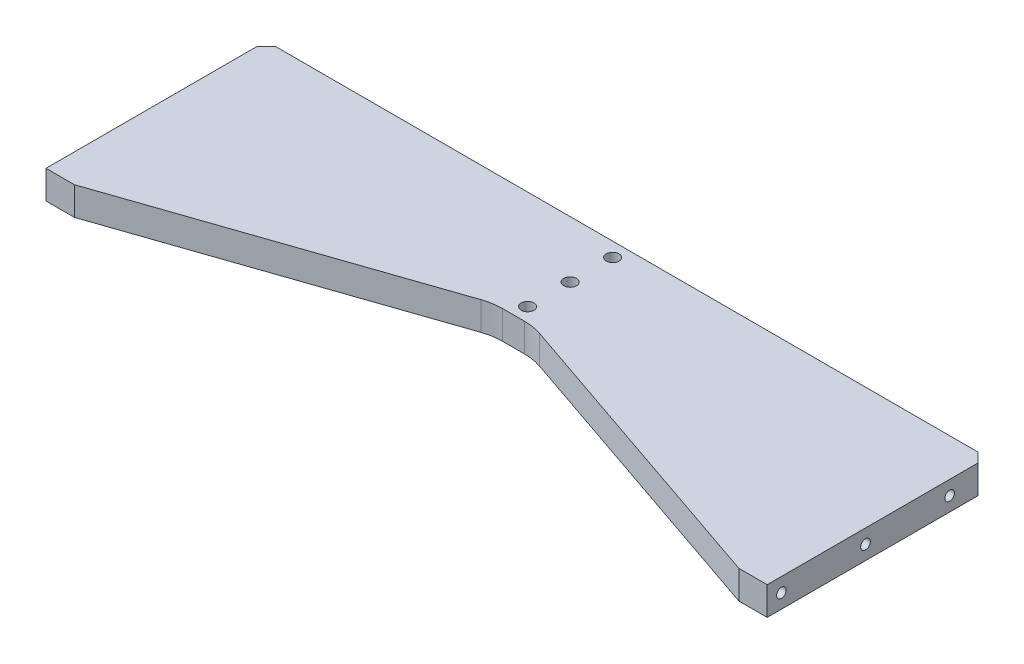
from build123d import *

# Parameters (mm, degrees)
SKETCH_1_W                = 763
SKETCH_1_H                = 233
EXTRUDE_1_DEPTH           = 30
CHAMFER_1_SIZE            = 10
CUT_EXTRUDE_1_DEPTH       = 401.018124589
CUT_EXTRUDE_1_DEPTH_BACK  = 30
FILLET_1_R                = 60
HOLE_WIZARD_1_D           = 13.5
HOLE_WIZARD_1_CBORE_D     = 20
HOLE_WIZARD_1_CBORE_DEPTH = 13
HOLE_WIZARD_M12_1_D       = 10.2
HOLE_WIZARD_M12_1_DEPTH   = 29.25
HOLE_WIZARD_M12_1_TIP     = 3.064389157
HOLE_WIZARD_M12_2_D       = 10.2
HOLE_WIZARD_M12_2_DEPTH   = 29.25
HOLE_WIZARD_M12_2_TIP     = 3.064389157
HOLE_WIZARD_M12_3_D       = 10.2
HOLE_WIZARD_M12_3_DEPTH   = 29.25
HOLE_WIZARD_M12_3_TIP     = 3.064389157


with BuildPart() as part:
    # 草图1 → 凸台-拉伸1 (new body)
    with BuildSketch(Plane(origin=(0, 0, 0), x_dir=(1, 0, 0), z_dir=(0, 1, 0))):
        Rectangle(SKETCH_1_W, SKETCH_1_H)
    extrude(amount=EXTRUDE_1_DEPTH)

    # 倒角1
    chamfer_1_edges = [part.edges().sort_by_distance(p)[0] for p in [
        (-381.5, 15, -116.5),
        (381.5, 15, -116.5),
    ]]
    chamfer(chamfer_1_edges, length=CHAMFER_1_SIZE)

    # 草图2 → 切除-拉伸1 (cut, two sides: drawn at the far end of the back side and taken through both)
    with BuildSketch(Plane(origin=(0, 30, 0), x_dir=(1, 0, 0), z_dir=(0, 1, 0)).offset(-CUT_EXTRUDE_1_DEPTH_BACK)):
        Polygon((-1816.285660926, -618.078120257), (-351.5, -116.5), (-21.5, -3.5), (21.5, -3.5), (351.5, -116.5), (1816.285660926, -618.078120257), (1816.285660926, -3714.642437803), (-1816.285660926, -3714.642437803), align=None)
    extrude(amount=CUT_EXTRUDE_1_DEPTH + CUT_EXTRUDE_1_DEPTH_BACK, mode=Mode.SUBTRACT)

    # 圆角1
    fillet_1_edges = [part.edges().sort_by_distance(p)[0] for p in [
        (21.5, 15, 3.5),
        (-21.5, 15, 3.5),
    ]]
    fillet(fillet_1_edges, radius=FILLET_1_R)

    # 打孔尺寸(%根据)内六角圆柱头螺钉的类型1 (through all)
    with Locations(Plane(origin=(0, 0, 0), x_dir=(-1, 0, 0), z_dir=(0, -1, 0))):
        with Locations((0, 11.5), (0, 56.5), (0, 101.5)):
            CounterBoreHole(HOLE_WIZARD_1_D / 2, HOLE_WIZARD_1_CBORE_D / 2, HOLE_WIZARD_1_CBORE_DEPTH)

    # M12 螺纹孔1
    with Locations(Plane(origin=(0, 0, -116.5), x_dir=(-1, 0, 0), z_dir=(0, 0, -1))):
        with Locations((351.5, 15), (251.071428571, 15), (150.642857143, 15), (50.214285714, 15), (-50.214285714, 15), (-150.642857143, 15), (-251.071428571, 15), (-351.5, 15)):
            Hole(HOLE_WIZARD_M12_1_D / 2, depth=HOLE_WIZARD_M12_1_DEPTH)
            with Locations((0, 0, -(HOLE_WIZARD_M12_1_DEPTH + HOLE_WIZARD_M12_1_TIP / 2))):  # 118° drill point
                Cone(0, HOLE_WIZARD_M12_1_D / 2, HOLE_WIZARD_M12_1_TIP, mode=Mode.SUBTRACT)

    # M12 螺纹孔2
    with Locations(Plane.ZY.offset(381.5)):
        with Locations((-76.5, 15), (12.5, 15), (101.5, 15)):
            Hole(HOLE_WIZARD_M12_2_D / 2, depth=HOLE_WIZARD_M12_2_DEPTH)
            with Locations((0, 0, -(HOLE_WIZARD_M12_2_DEPTH + HOLE_WIZARD_M12_2_TIP / 2))):  # 118° drill point
                Cone(0, HOLE_WIZARD_M12_2_D / 2, HOLE_WIZARD_M12_2_TIP, mode=Mode.SUBTRACT)

    # M12 螺纹孔3
    with Locations(Plane(origin=(381.5, 0, 0), x_dir=(0, 0, -1), z_dir=(1, 0, 0))):
        with Locations((76.5, 15), (-12.5, 15), (-101.5, 15)):
            Hole(HOLE_WIZARD_M12_3_D / 2, depth=HOLE_WIZARD_M12_3_DEPTH)
            with Locations((0, 0, -(HOLE_WIZARD_M12_3_DEPTH + HOLE_WIZARD_M12_3_TIP / 2))):  # 118° drill point
                Cone(0, HOLE_WIZARD_M12_3_D / 2, HOLE_WIZARD_M12_3_TIP, mode=Mode.SUBTRACT)


solid = part.part
